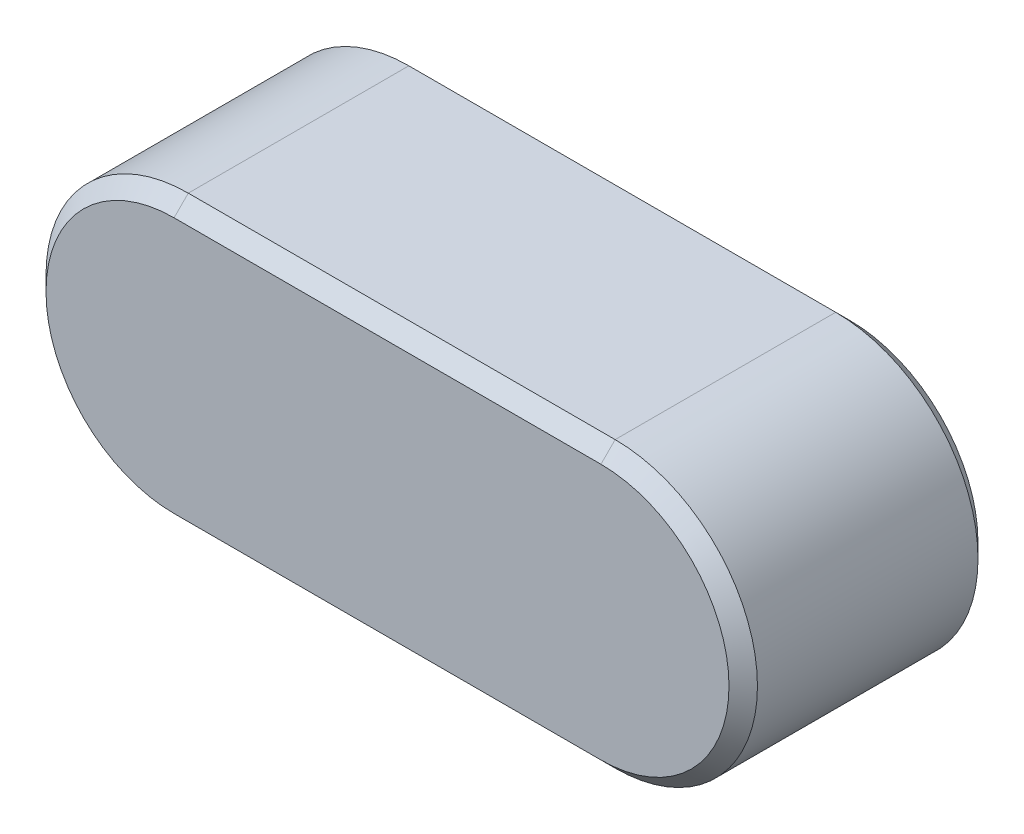
SolidWorks part; units mm, degrees
ref_plane "Front" through (0, 0, 0) normal (0, 0, 1) x (1, 0, 0)
ref_plane "Top" through (0, 0, 0) normal (0, 1, 0) x (1, 0, 0)
ref_plane "Right" through (0, 0, 0) normal (1, 0, 0) x (0, 0, -1)
sketch "Sketch1" plane through (0, 0, 0) normal (0, 0, 1) x (1, 0, 0)
  line L0 (-12, 4) -> (0, 4)
  line L1 (0, -4) -> (-12, -4)
  arc A0 (0, 4) -> (0, -4) centre (0, 0) cw
  arc A1 (-12, -4) -> (-12, 4) centre (-12, 0) cw
  dimension "L" = 20
  dimension "b" = 8
extrude "BaseKey" add sketch "Sketch1" along normal mid plane 7
sketch "Sketch2" plane through (0, 0, 0) normal (0, 0, 1) x (1, 0, 0)
  line L1 (-16, 4) -> (4, 4)
  line L2 (-16, 4) -> (-16, -4)
  line L3 (-16, -4) -> (4, -4)
  line L4 (4, 4) -> (4, -4)
  line L6 (0, -4) -> (-12, -4) construction
  line L7 (-12, 4) -> (0, 4) construction
  arc A2 (0, -4) -> (0, 4) centre (0, 0) ccw construction
  arc A3 (-12, 4) -> (-12, -4) centre (-12, 0) ccw construction
extrude "Extrude1" [suppressed] add sketch "Sketch2" along normal mid plane 7
sketch "Sketch3" plane through (0, 0, 0) normal (0, 0, 1) x (1, 0, 0)
  line L0 (4, 4) -> (-12, 4)
  line L1 (-12, -4) -> (4, -4)
  line L2 (4, -4) -> (4, 4)
  line L5 (-12, 4) -> (0, 4) construction
  arc A0 (-12, 4) -> (-12, -4) centre (-12, 0) ccw
  arc A1 (0, -4) -> (0, 4) centre (0, 0) ccw construction
  arc A4 (-12, 4) -> (-12, -4) centre (-12, 0) ccw construction
extrude "Extrude2" [suppressed] add sketch "Sketch3" along normal mid plane 7
chamfer "Chamfer1" distance 0.4 angle 45 8 edges at (4, 0, -3.5) (-6, -4, -3.5) (-16, 0, -3.5) (-6, 4, -3.5) (-16, 0, 3.5) (-6, -4, 3.5) (4, 0, 3.5) (-6, 4, 3.5)
equation "\"D1@Extrude1\"=\"h@BaseKey\""
equation "\"D1@Extrude2\"=\"h@BaseKey\""
